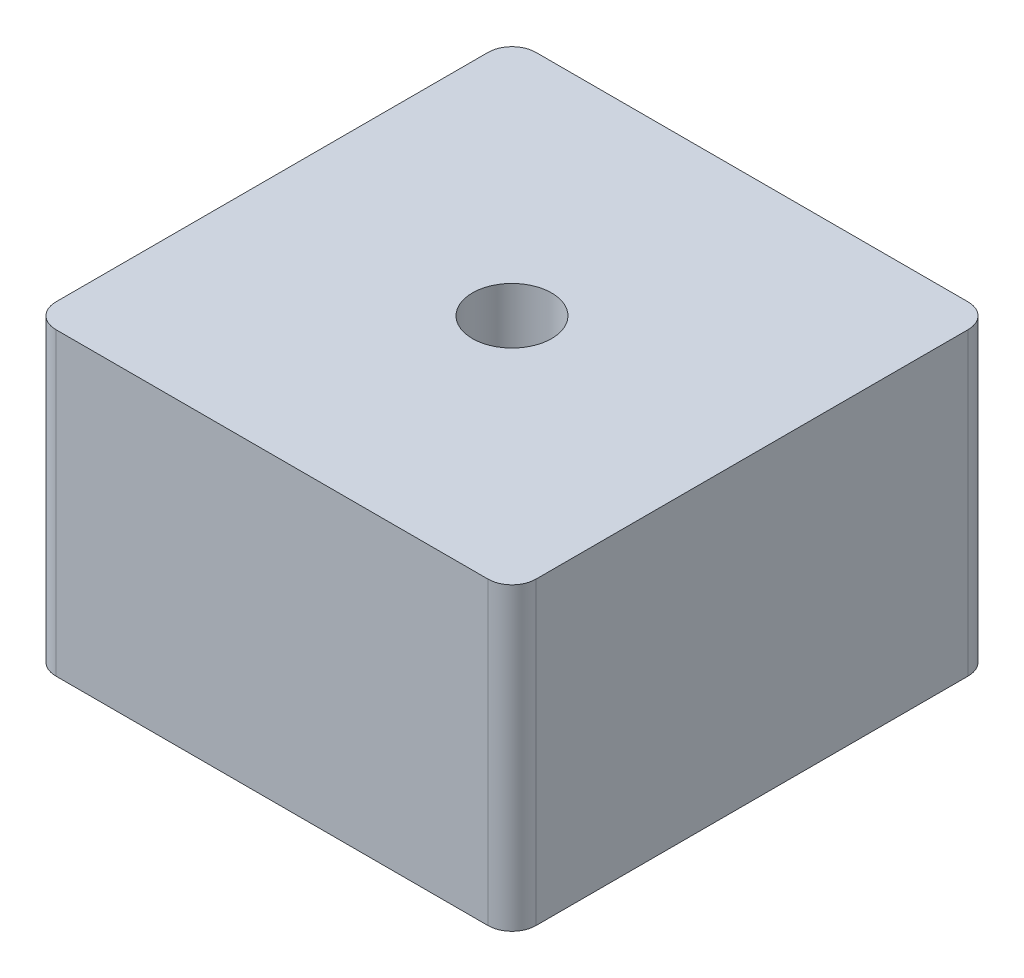
SolidWorks part; units mm, degrees
ref_plane "Front Plane" through (0, 0, 0) normal (0, 0, 1) x (1, 0, 0)
ref_plane "Top Plane" through (0, 0, 0) normal (0, 1, 0) x (1, 0, 0)
ref_plane "Right Plane" through (0, 0, 0) normal (1, 0, 0) x (0, 0, -1)
other "Configuration Table"
sketch "Sketch1" plane through (0, 0, 0) normal (0, 1, 0) x (1, 0, 0)
  line L1 (-10, 10) -> (10, 10)
  line L2 (-10, 10) -> (-10, -10)
  line L3 (-10, -10) -> (10, -10)
  line L4 (10, 10) -> (10, -10)
  line L5 (-10, 10) -> (10, -10) construction
  line L6 (-10, -10) -> (10, 10) construction
  point P0 (0, 0)
  dimension "D1" = 20
  dimension "D2" = 20
extrude "Boss-Extrude1" add sketch "Sketch1" along normal blind 12.5
sketch "Sketch2" plane through (0, 12.5, 0) normal (0, 1, 0) x (1, 0, 0)
  point P0 (0, 0)
hole_wizard "M4 Tapped Hole1" positions "Sketch2" profile "Sketch3" tap size "M4" standard "GB" end condition through all
sketch "Sketch3" plane through (0, 12.5, 0) normal (1, 0, 0) x (0, 0, 1)
  line L0 (0, 0) -> (0, 12.5)
  line L1 (0, 12.5) -> (1.65, 12.5)
  line L2 (1.65, 12.5) -> (1.65, 0)
  line L5 (1.65, 0) -> (0, 0)
  line L11 (0, -6.35) -> (0, 107.95) construction
  dimension "通孔螺纹孔钻头直径" = 3.3
  dimension "通孔螺纹孔钻头深度" = 12.5
cosmetic thread "Cosmetic thread 1"
fillet "Fillet1" radius 1 4 edges at (-10, 6.25, -10) (10, 6.25, -10) (10, 6.25, 10) (-10, 6.25, 10)
